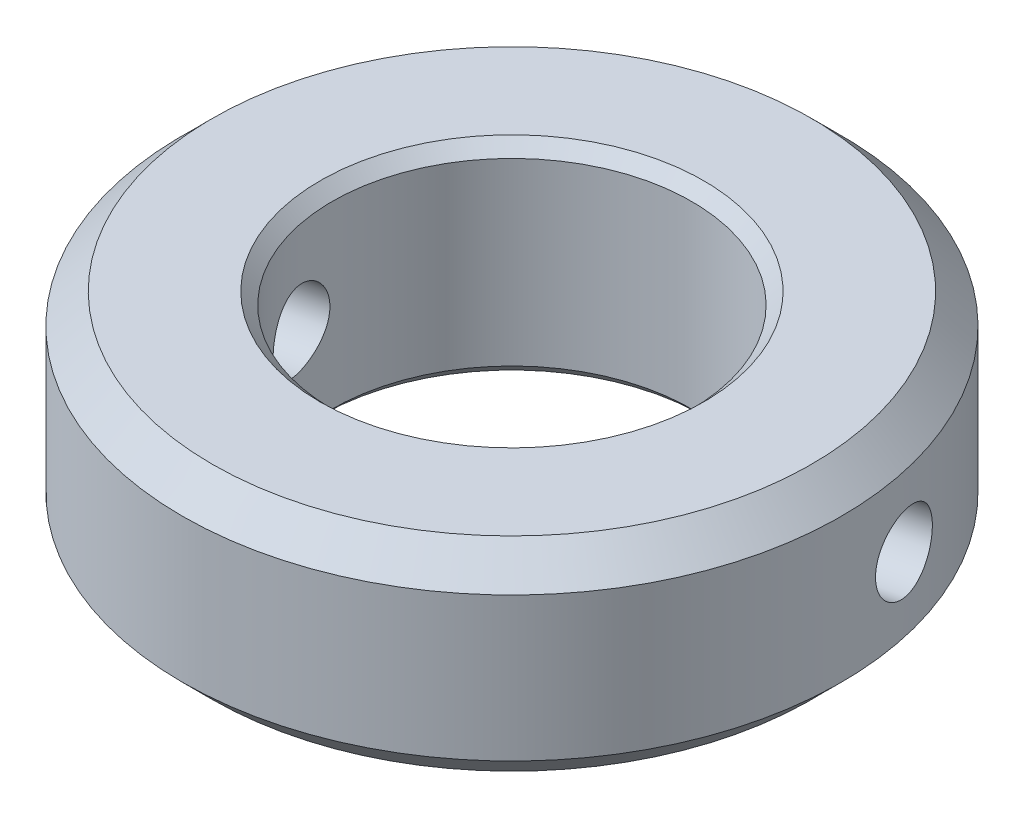
SolidWorks part; units mm, degrees
ref_plane "Front Plane" through (0, 0, 0) normal (0, 0, 1) x (1, 0, 0)
ref_plane "Top Plane" through (0, 0, 0) normal (0, 1, 0) x (1, 0, 0)
ref_plane "Right Plane" through (0, 0, 0) normal (1, 0, 0) x (0, 0, -1)
sketch "Sketch1" plane through (0, 0, 0) normal (0, 1, 0) x (1, 0, 0)
  circle A0 centre (0, 0) radius 30
  circle A1 centre (0, 0) radius 55
  dimension "D1" = 60
  dimension "D2" = 110
extrude "Boss-Extrude1" add sketch "Sketch1" along normal blind 34
hole_wizard "Ø17.0 (17) Diameter Hole1" positions "3DSketch1" profile "Sketch2" hole size "Ø17.0" standard "GB" end condition through all
sketch3d "3DSketch1"
  point P0 (53.6236, 17, -12.2276)
  dimension "D1" = 17
sketch "Sketch2" plane through (53.6236, 17, -12.2276) normal (0, 1, 0) x (-0.2223, 0, -0.975)
  line L0 (0, 0) -> (0, 120.8511)
  line L1 (0, 120.8511) -> (6.3, 120.8511)
  line L2 (6.3, 120.8511) -> (6.3, 0)
  line L5 (6.3, 0) -> (0, 0)
  line L11 (0, -6.35) -> (0, 107.95) construction
  dimension "通孔孔直径" = 12.6
  dimension "通孔孔深度" = 120.8511
chamfer "Chamfer1" distance 5 angle 45 2 edges at (0, 0, 55) (0, 34, 55)
chamfer "Chamfer2" distance 2 angle 45 2 edges at (0, 0, 30) (0, 34, 30)
